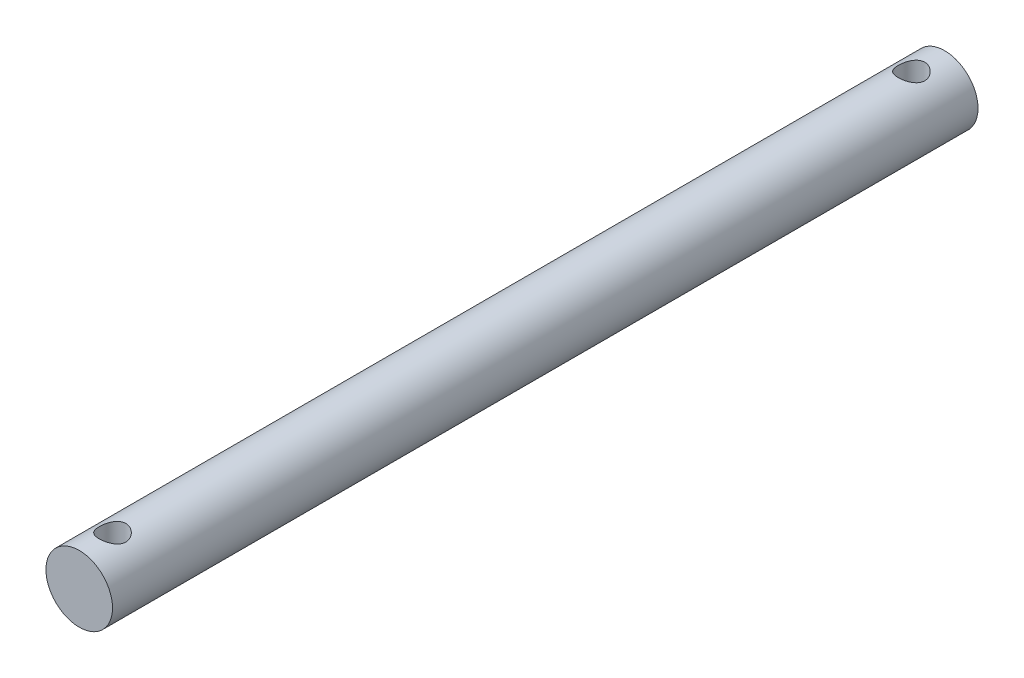
from build123d import *

# Parameters (mm, degrees)
SKETCH_1_R          = 5
EXTRUDE_1_DEPTH     = 65
SKETCH_2_R          = 2
CUT_EXTRUDE_1_DEPTH = 10


with BuildPart() as part:
    # 草图1 → 凸台-拉伸1 (new, symmetric)
    with BuildSketch(Plane.XY):
        Circle(SKETCH_1_R)
    extrude(amount=EXTRUDE_1_DEPTH, both=True)

    # 草图2 → 切除-拉伸1 (cut)
    with BuildSketch(Plane(origin=(0, 5, 0), x_dir=(1, 0, 0), z_dir=(0, 1, 0))):
        with Locations(Location((0, -60, 0), (0, 0, 270))):
            Circle(SKETCH_2_R)
        with Locations(Location((0, 60, 0), (0, 0, 270))):
            Circle(SKETCH_2_R)
    extrude(amount=-CUT_EXTRUDE_1_DEPTH, mode=Mode.SUBTRACT)


solid = part.part
